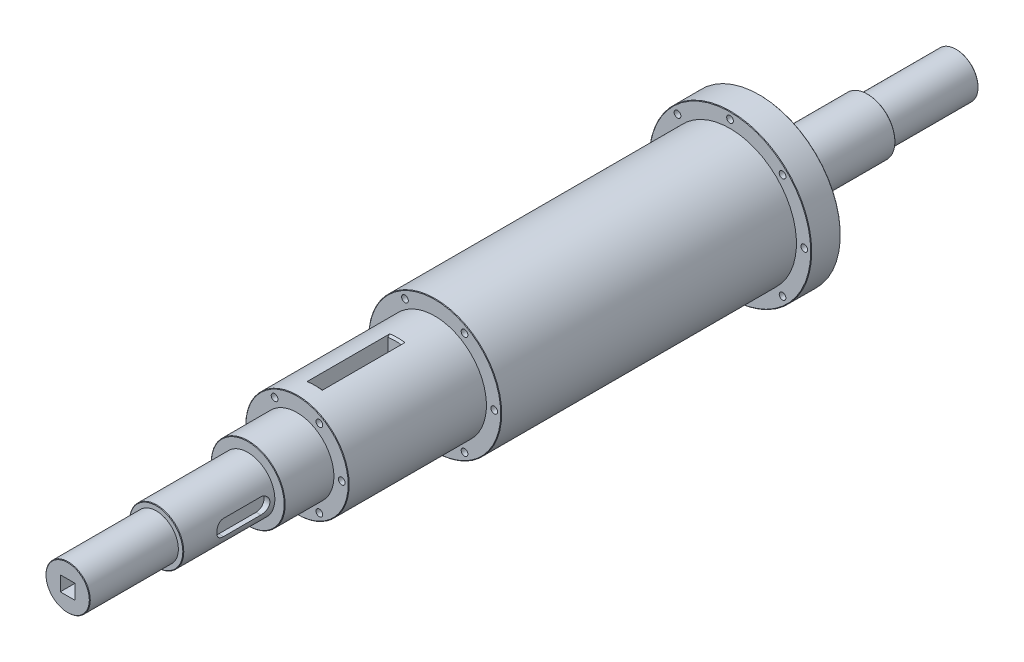
SolidWorks part; units mm, degrees
material "合金钢"
ref_plane "前视基准面" through (0, 0, 0) normal (0, 0, 1) x (1, 0, 0)
ref_plane "上视基准面" through (0, 0, 0) normal (0, 1, 0) x (1, 0, 0)
ref_plane "右视基准面" through (0, 0, 0) normal (1, 0, 0) x (0, 0, -1)
sketch "草图2" plane through (0, 0, 0) normal (0, 1, 0) x (1, 0, 0)
  line L0 (0, 0) -> (0, -34294.6447) construction
  line L1 (0, 563.143) -> (-22.5, 563.143)
  line L2 (-22.5, 563.143) -> (-22.5, 473.143)
  line L3 (-28, 363.143) -> (-82.5, 363.143)
  line L5 (-67.5, 33.143) -> (-52.5, 33.143)
  line L10 (-52.5, 33.143) -> (-52.5, -106.857)
  line L11 (-52.5, -106.857) -> (-37.5, -106.857)
  line L16 (-37.5, -106.857) -> (-37.5, -156.857)
  line L17 (-37.5, -156.857) -> (-27.5, -156.857)
  line L18 (-22.5, -249.857) -> (-22.5, -339.857)
  line L19 (-22.5, -339.857) -> (0, -339.857)
  line L20 (0, -339.857) -> (0, 563.143)
  line L21 (-67.5, 33.143) -> (-67.5, 333.143)
  line L22 (-67.5, 333.143) -> (-82.5, 333.143)
  line L23 (-82.5, 333.143) -> (-82.5, 363.143)
  line L24 (-22.5, 473.143) -> (-28, 473.143)
  line L25 (-28, 473.143) -> (-28, 363.143)
  line L26 (-22.5, -249.857) -> (-27.5, -249.857)
  line L27 (-27.5, -249.857) -> (-27.5, -156.857)
  dimension "D1" = 45
  dimension "D2" = 56
  dimension "D3" = 15
  dimension "D4" = 15
  dimension "D5" = 55
  dimension "D6" = 45
  dimension "D7" = 15
  dimension "D8" = 140
  dimension "D9" = 300
  dimension "D10" = 363.143
  dimension "D11" = 233
  dimension "D12" = 30
  dimension "D13" = 50
  dimension "D14" = 110
  dimension "D15" = 90
  dimension "D16" = 90
  dimension "D17" = 75
revolve "旋转1" add sketch "草图2" angle 360 about L0
sketch "草图3" plane through (0, 0, -563.143) normal (0, 0, -1) x (-1, 0, 0)
  line L1 (-7.5, 7.5) -> (7.5, 7.5)
  line L2 (-7.5, 7.5) -> (-7.5, -7.5)
  line L3 (-7.5, -7.5) -> (7.5, -7.5)
  line L4 (7.5, 7.5) -> (7.5, -7.5)
  line L5 (-7.5, 7.5) -> (7.5, -7.5) construction
  line L6 (-7.5, -7.5) -> (7.5, 7.5) construction
  point P0 (0, 0)
  dimension "D1" = 15
  dimension "D2" = 15
extrude "切除-拉伸1" cut sketch "草图3" against normal through all
sketch "草图4" plane through (0, 0, 0) normal (0, 1, 0) x (1, 0, 0)
  line L0 (-67.5, 33.143) -> (67.5, 33.143) construction
  line L1 (7.7, -6.857) -> (-7.7, -6.857)
  line L2 (7.7, -6.857) -> (7.7, -86.857)
  line L3 (7.7, -86.857) -> (-7.7, -86.857)
  line L4 (-7.7, -6.857) -> (-7.7, -86.857)
  dimension "D1" = 7.7
  dimension "D2" = 7.7
  dimension "D3" = 40
  dimension "D4" = 80
extrude "切除-拉伸2" cut sketch "草图4" against normal through all both and the other way through all
chamfer "倒角1" distance 2 angle 45 4 edges at (0, -52.5, 86.857) (0, 52.5, 86.857) (0, -52.5, 6.857) (0, 52.5, 6.857)
hole_wizard "M8 螺纹孔1" positions "草图5" profile "草图6" tap size "M8" standard "GB"
sketch "草图5" plane through (0, 0, 106.857) normal (0, 0, 1) x (1, 0, 0)
  circle A1 centre (0, 0) radius 52.5 construction
  point P2 (-45.5, 0)
  dimension "D1" = 7
sketch "草图6" plane through (-45.5, 0, 106.857) normal (1, 0, 0) x (0, -1, 0)
  line L0 (0, 0) -> (0, 21.7929)
  line L1 (0, 21.7929) -> (3.4, 19.75)
  line L2 (3.4, 19.75) -> (3.4, 0)
  line L5 (3.4, 0) -> (0, 0)
  line L10 (0, 21.7929) -> (-3.4, 19.75) construction
  line L11 (0, -6.35) -> (0, 107.95) construction
  dimension "螺纹孔钻头直径" = 6.8
  dimension "螺纹孔钻头深度" = 19.75
  dimension "导头角度" = 118
cosmetic thread "孔螺蚊线1" parameters "D1"=16, "D2"=8
pattern_circular "阵列(圆周)1" count 6 over 360 about axis through (0, 0, 0) along (0, 0, 1) of "M8 螺纹孔1"
hole_wizard "M8 螺纹孔2" positions "草图8" profile "草图9" tap size "M8" standard "GB"
sketch "草图8" plane through (0, 0, -33.143) normal (0, 0, 1) x (1, 0, 0)
  circle A2 centre (0, 0) radius 67.5 construction
  point P0 (60.5, 0)
  dimension "D1" = 7
sketch "草图9" plane through (60.5, 0, -33.143) normal (1, 0, 0) x (0, -1, 0)
  line L0 (0, 0) -> (0, 21.7929)
  line L1 (0, 21.7929) -> (3.4, 19.75)
  line L2 (3.4, 19.75) -> (3.4, 0)
  line L5 (3.4, 0) -> (0, 0)
  line L10 (0, 21.7929) -> (-3.4, 19.75) construction
  line L11 (0, -6.35) -> (0, 107.95) construction
  dimension "螺纹孔钻头直径" = 6.8
  dimension "螺纹孔钻头深度" = 19.75
  dimension "导头角度" = 118
cosmetic thread "孔螺蚊线2" parameters "D1"=16, "D2"=8
pattern_circular "阵列(圆周)2" count 6 over 360 about axis through (0, 0, 0) along (0, 0, 1) of "M8 螺纹孔2"
hole_wizard "M8 螺纹孔3" positions "草图10" profile "草图11" tap size "M8" standard "GB"
sketch "草图10" plane through (0, 0, -333.143) normal (0, 0, 1) x (1, 0, 0)
  circle A0 centre (0, 0) radius 82.5 construction
  point P0 (-75.5, 0)
  dimension "D1" = 7
sketch "草图11" plane through (-75.5, 0, -333.143) normal (1, 0, 0) x (0, -1, 0)
  line L0 (0, 0) -> (0, 21.7929)
  line L1 (0, 21.7929) -> (3.4, 19.75)
  line L2 (3.4, 19.75) -> (3.4, 0)
  line L5 (3.4, 0) -> (0, 0)
  line L10 (0, 21.7929) -> (-3.4, 19.75) construction
  line L11 (0, -6.35) -> (0, 107.95) construction
  dimension "螺纹孔钻头直径" = 6.8
  dimension "螺纹孔钻头深度" = 19.75
  dimension "导头角度" = 118
cosmetic thread "孔螺蚊线3" parameters "D1"=16, "D2"=8
pattern_circular "阵列(圆周)3" count 8 over 360 about axis through (0, 0, 0) along (0, 0, 1) of "M8 螺纹孔3"
chamfer "倒角2" distance 0.5 angle 45 9 edges at (-22.5, 0, -563.143) (-28, 0, -473.143) (-82.5, 0, -363.143) (-82.5, 0, -333.143) (-67.5, 0, -33.143) (-52.5, 0, 106.857) (-37.5, 0, 156.857) (-27.5, 0, 249.857) (-22.5, 0, 339.857)
chamfer "倒角3" distance 3 angle 60 4 edges at (7.5, 0, -563.143) (0, 7.5, -563.143) (-7.5, 0, -563.143) (0, -7.5, -563.143)
chamfer "倒角4" distance 3 angle 60 2 edges at (0, 7.5, 86.857) (0, -7.5, 86.857)
ref_plane "基准面1" through (27.5, 0, 0) normal (1, 0, 0) x (0, 0, -1)
sketch "草图12" plane through (27.5, 0, 0) normal (1, 0, 0) x (0, 0, -1)
  line L0 (-169.857, 0) -> (-207.857, 0) construction
  line L1 (-169.857, -8) -> (-207.857, -8)
  line L2 (-169.857, 8) -> (-207.857, 8)
  line L6 (-156.857, 27.5) -> (-156.857, -27.5) construction
  arc A0 (-169.857, -8) -> (-169.857, 8) centre (-169.857, 0) ccw
  arc A1 (-207.857, 8) -> (-207.857, -8) centre (-207.857, 0) ccw
  point P2 (-188.857, 0)
  dimension "D2" = 54
  dimension "D3" = 5
  dimension "D1" = 16
extrude "切除-拉伸3" cut sketch "草图12" against normal blind 6
